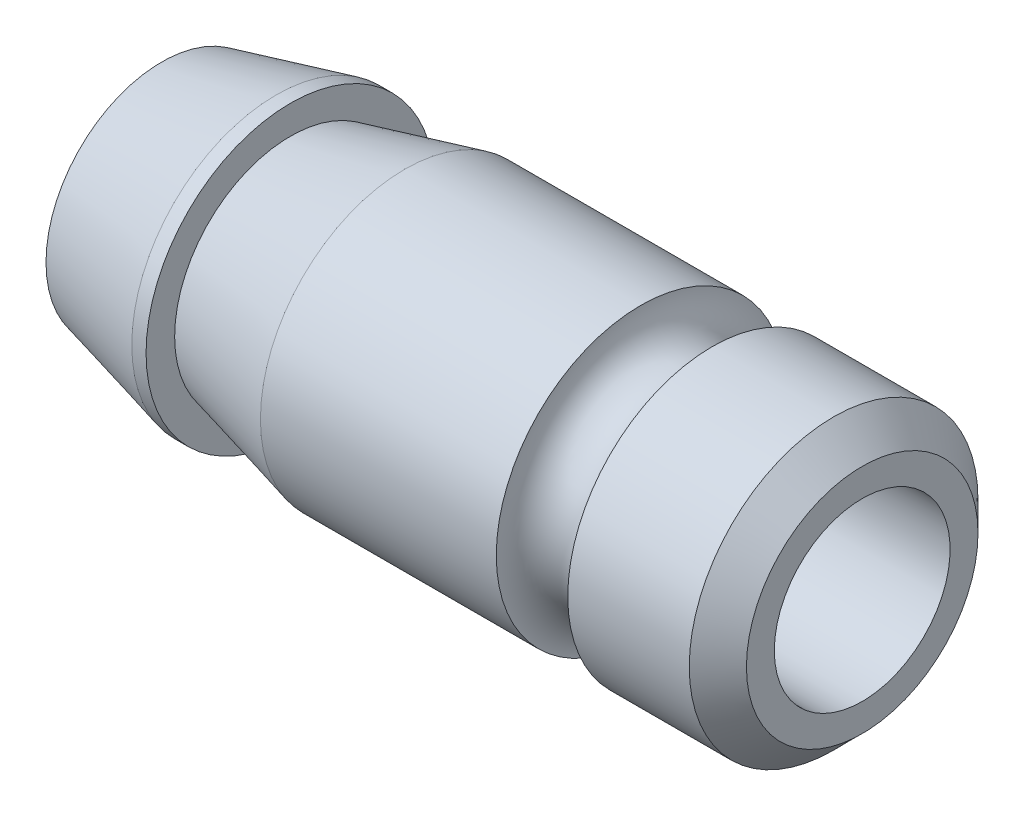
SolidWorks part; units mm, degrees
ref_plane "Front Plane" through (0, 0, 0) normal (0, 0, 1) x (1, 0, 0)
ref_plane "Top Plane" through (0, 0, 0) normal (0, 1, 0) x (1, 0, 0)
ref_plane "Right Plane" through (0, 0, 0) normal (1, 0, 0) x (0, 0, -1)
sketch "Sketch1" plane through (0, 0, 0) normal (0, 0, 1) x (1, 0, 0)
  line L0 (17, 10.1) -> (9, 8.1)
  line L1 (9, 10.1) -> (8, 10.1)
  line L2 (8, 10.1) -> (0, 8.1)
  line L3 (47, 10.1) -> (38.5, 10.1)
  line L4 (33.5, 10.1) -> (17, 10.1)
  line L5 (49, 8.1) -> (47, 10.1)
  line L6 (9, 8.1) -> (9, 10.1)
  line L7 (0, 8.1) -> (0, 0)
  line L8 (49, 8.1) -> (49, 0)
  line L9 (0, 0) -> (49, 0)
  arc A0 (33.5, 10.1) -> (38.5, 10.1) centre (36, 10.1) ccw
  dimension "D3" = 2.5
  dimension "D1" = 8.1
  dimension "D2" = 10.1
  dimension "D4" = 13
  dimension "D5" = 16.5
  dimension "D6" = 10.1
  dimension "D7" = 8.1
  dimension "D8" = 8
  dimension "D9" = 1
  dimension "D10" = 10.1
  dimension "D11" = 8
  dimension "D12" = 2
  dimension "D13" = 2
  dimension "D14" = 2
revolve "Revolve1" add sketch "Sketch1" angle 360 about L9
sketch "Sketch2" plane through (0, 0, 0) normal (-1, 0, 0) x (0, 0, 1)
  circle A0 centre (0, 0) radius 6.15
  dimension "D1" = 12.3
extrude "Cut-Extrude1" cut sketch "Sketch2" against normal blind 99
